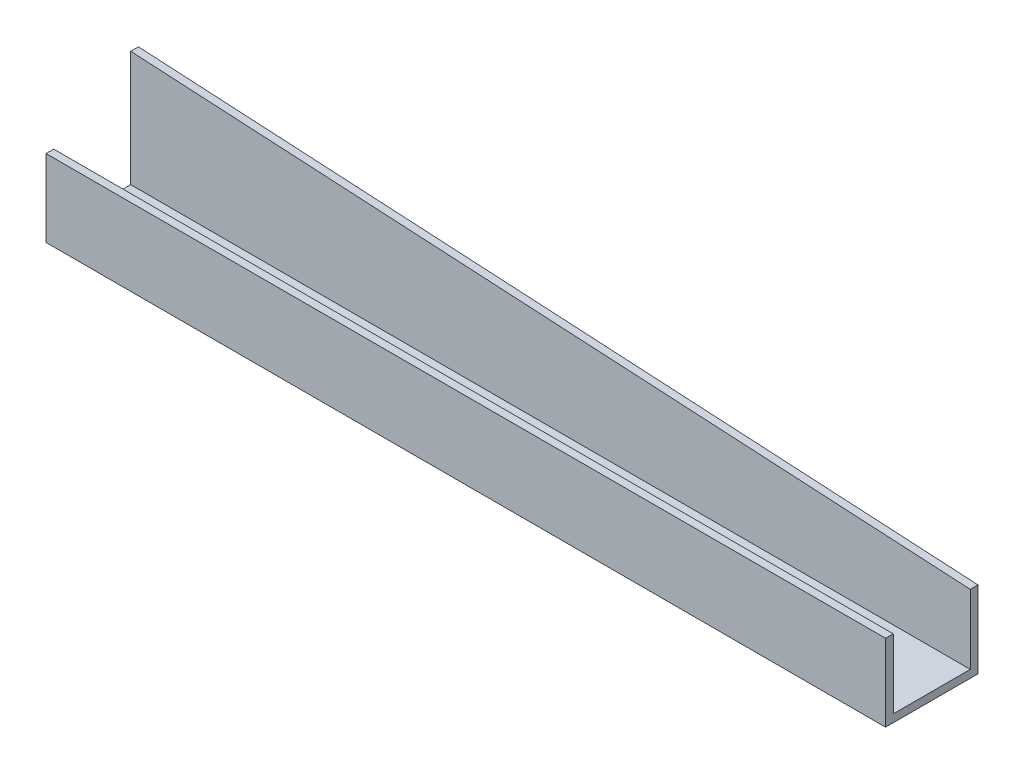
from build123d import *

# Parameters (mm, degrees)
EXTRUDE_1_DEPTH     = 60
SHELL_2_T           = -5
CUT_EXTRUDE_2_DEPTH = 38


with BuildPart() as part:
    # 草图1 → 凸台-拉伸1 (new body)
    with BuildSketch(Plane.XY):
        Polygon((0, 0), (0, -80), (545, -80), (545, -30), align=None)
    extrude(amount=EXTRUDE_1_DEPTH)

    # 抽壳2
    shell_2_openings = [part.faces().sort_by_distance(p)[0] for p in [
        (545, -55, 30),
        (0, -40, 30),
        (272.5, -15, 30),
    ]]
    offset(amount=SHELL_2_T, openings=shell_2_openings, kind=Kind.INTERSECTION)

    # 草图4 → 切除-拉伸2 (cut)
    with BuildSketch(Plane.XY.offset(60)):
        Polygon((545, -30), (0, -30), (0, 50.034428037), align=None)
    extrude(amount=-CUT_EXTRUDE_2_DEPTH, mode=Mode.SUBTRACT)


solid = part.part
